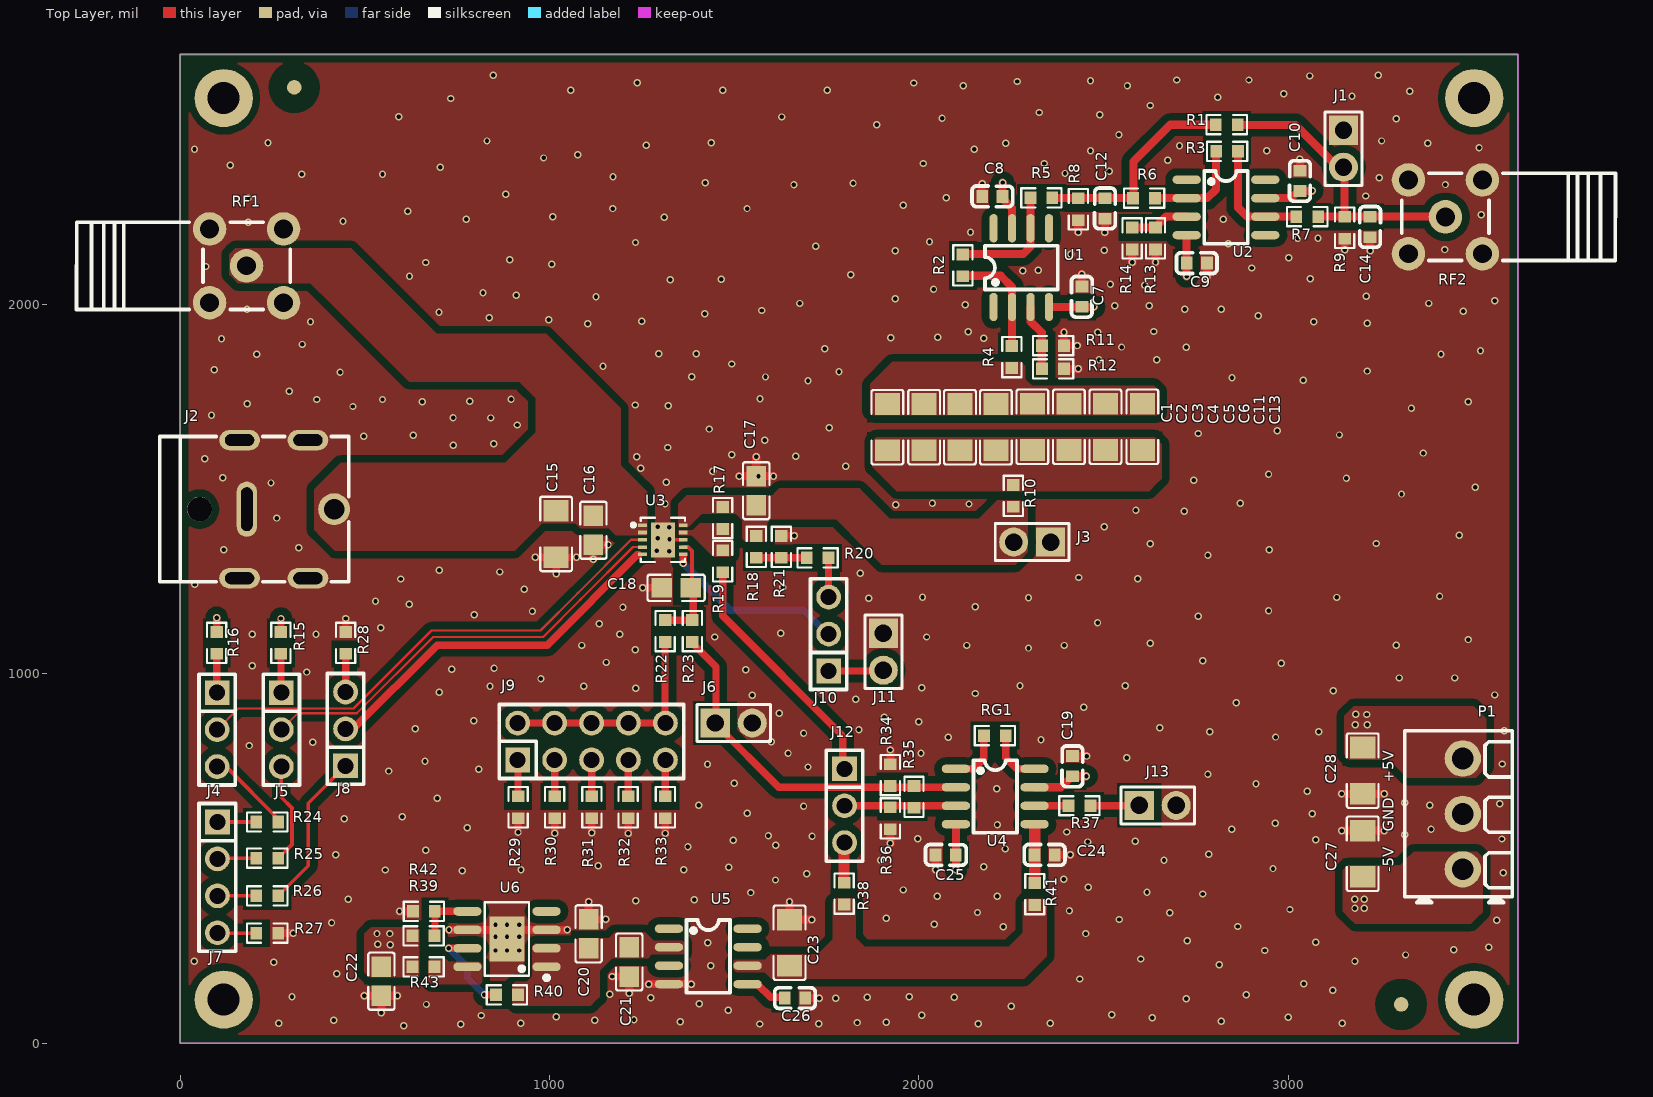
[diagram p0: Top Layer view]
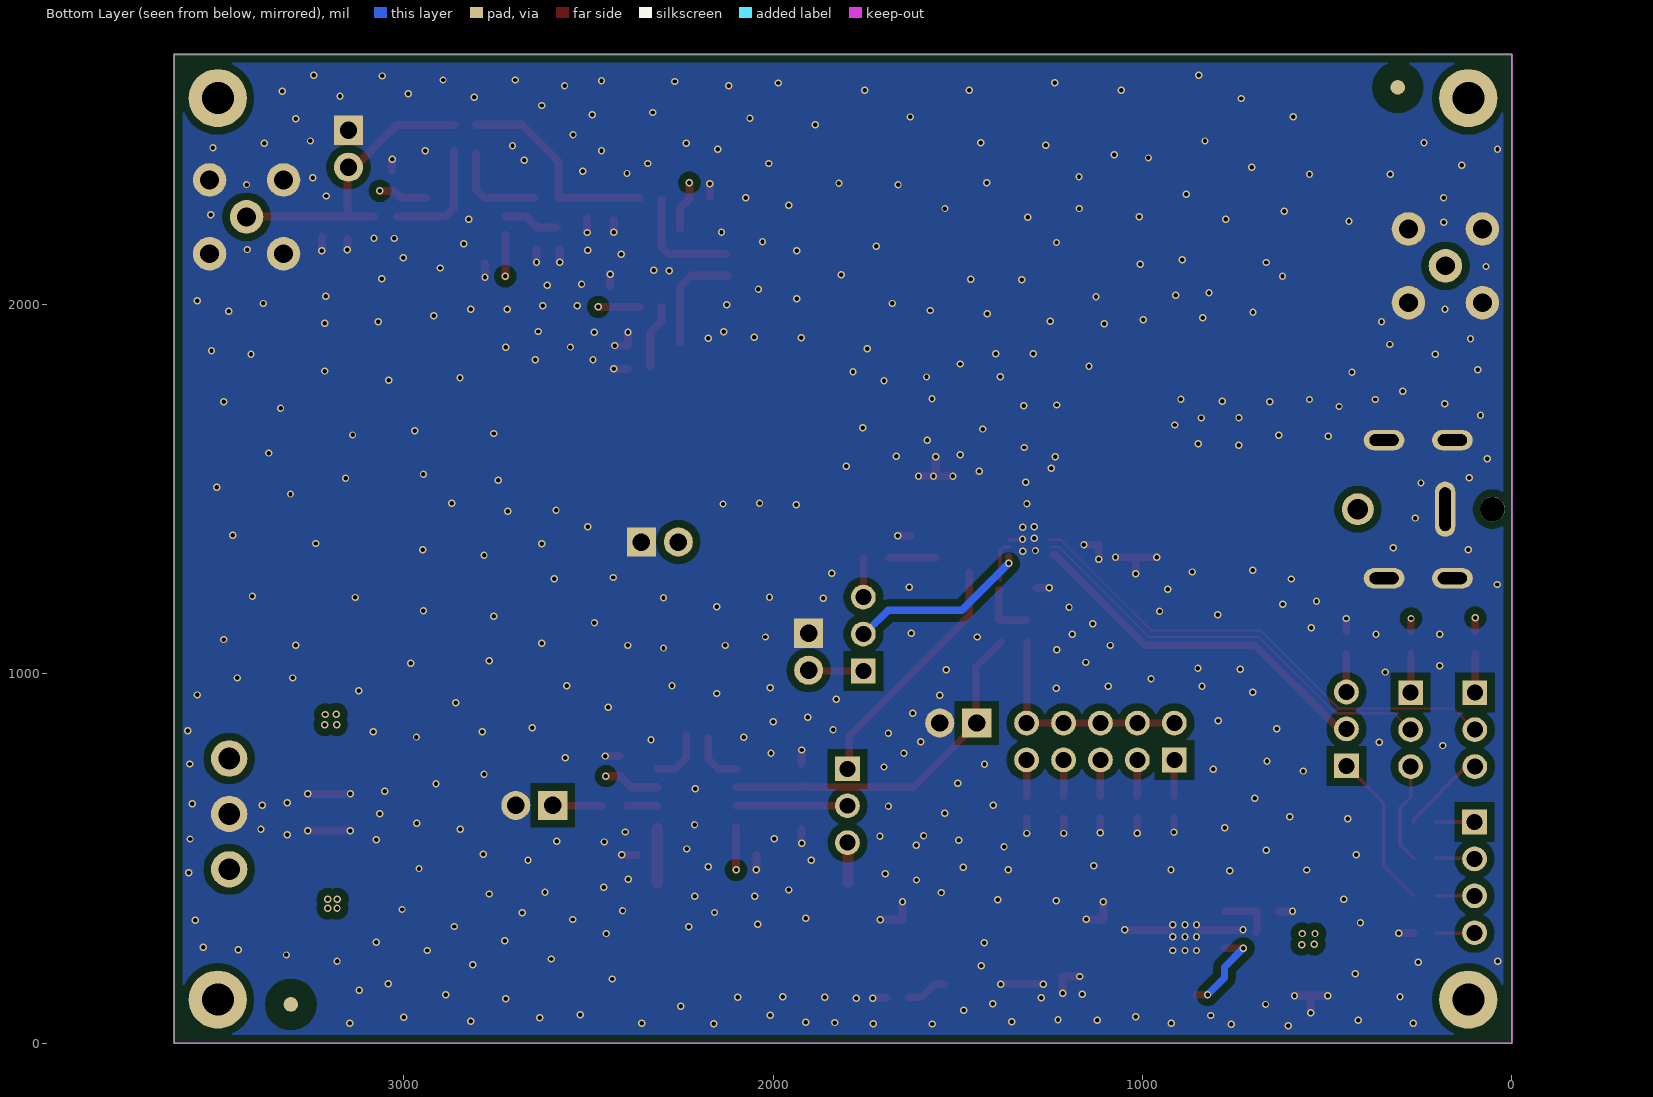
[diagram p1: Bottom Layer view, seen from below]
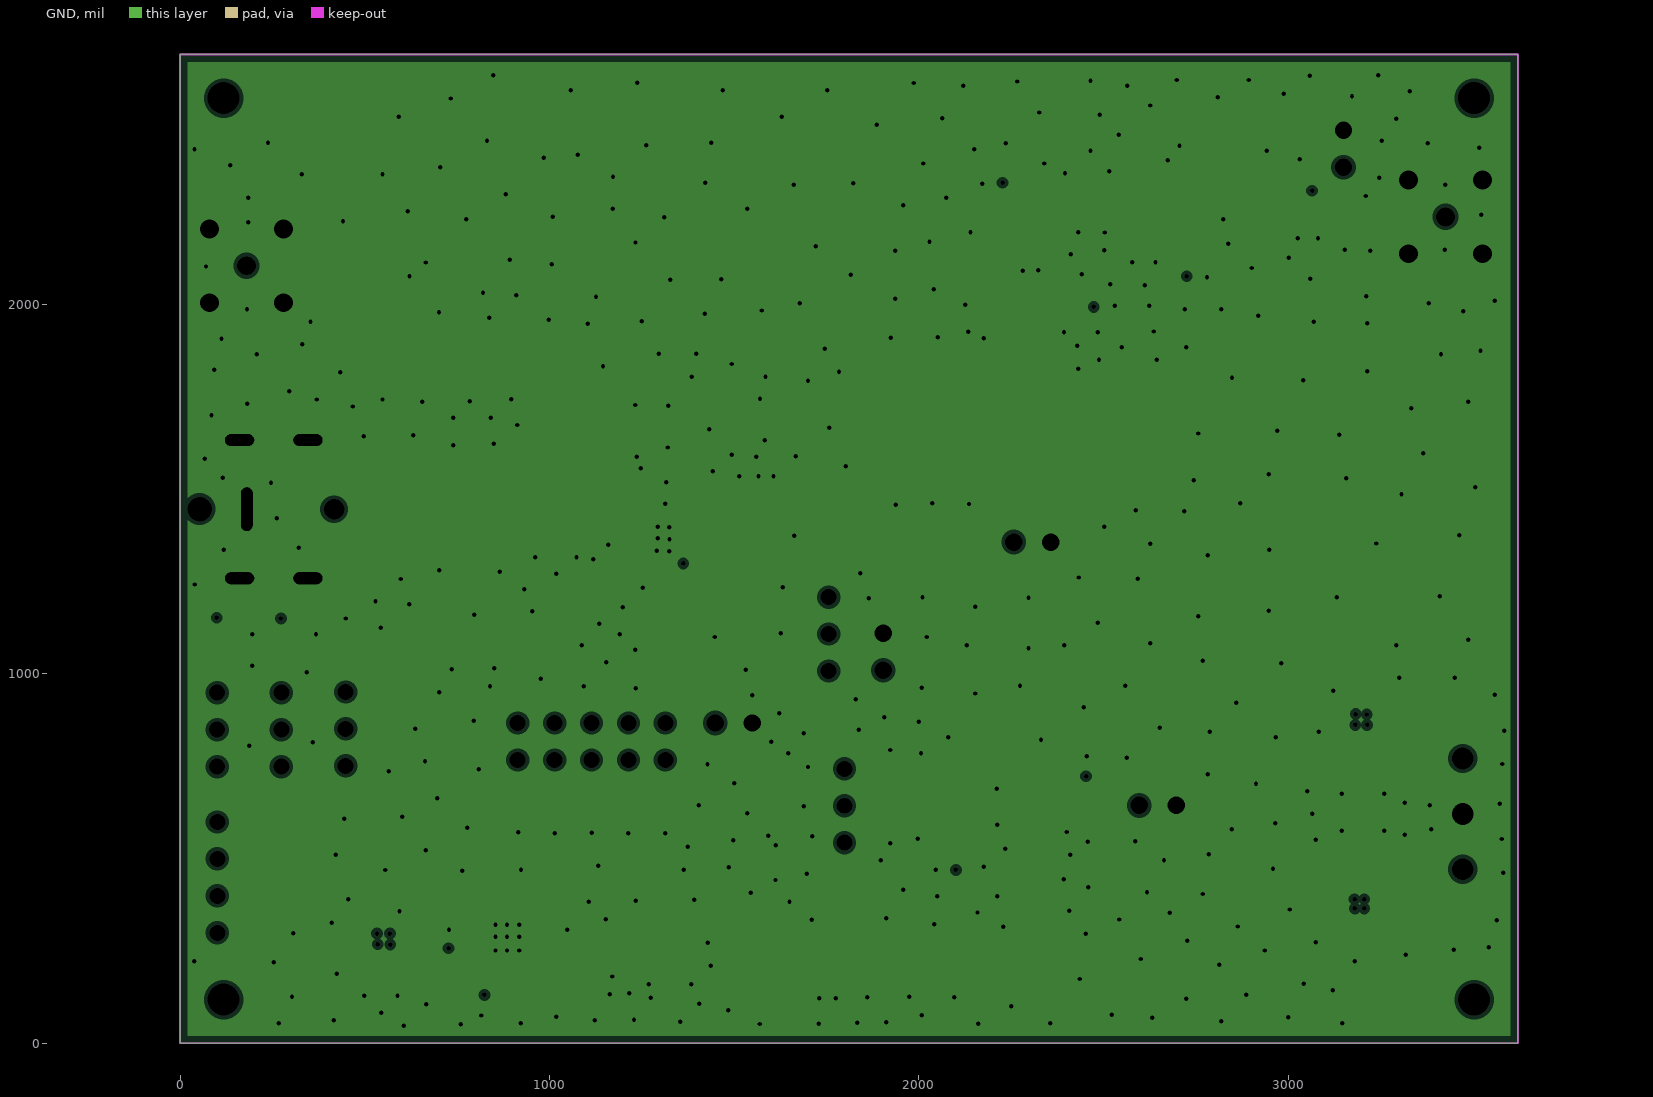
[diagram p2: GND, clearances drawn from the general rule]
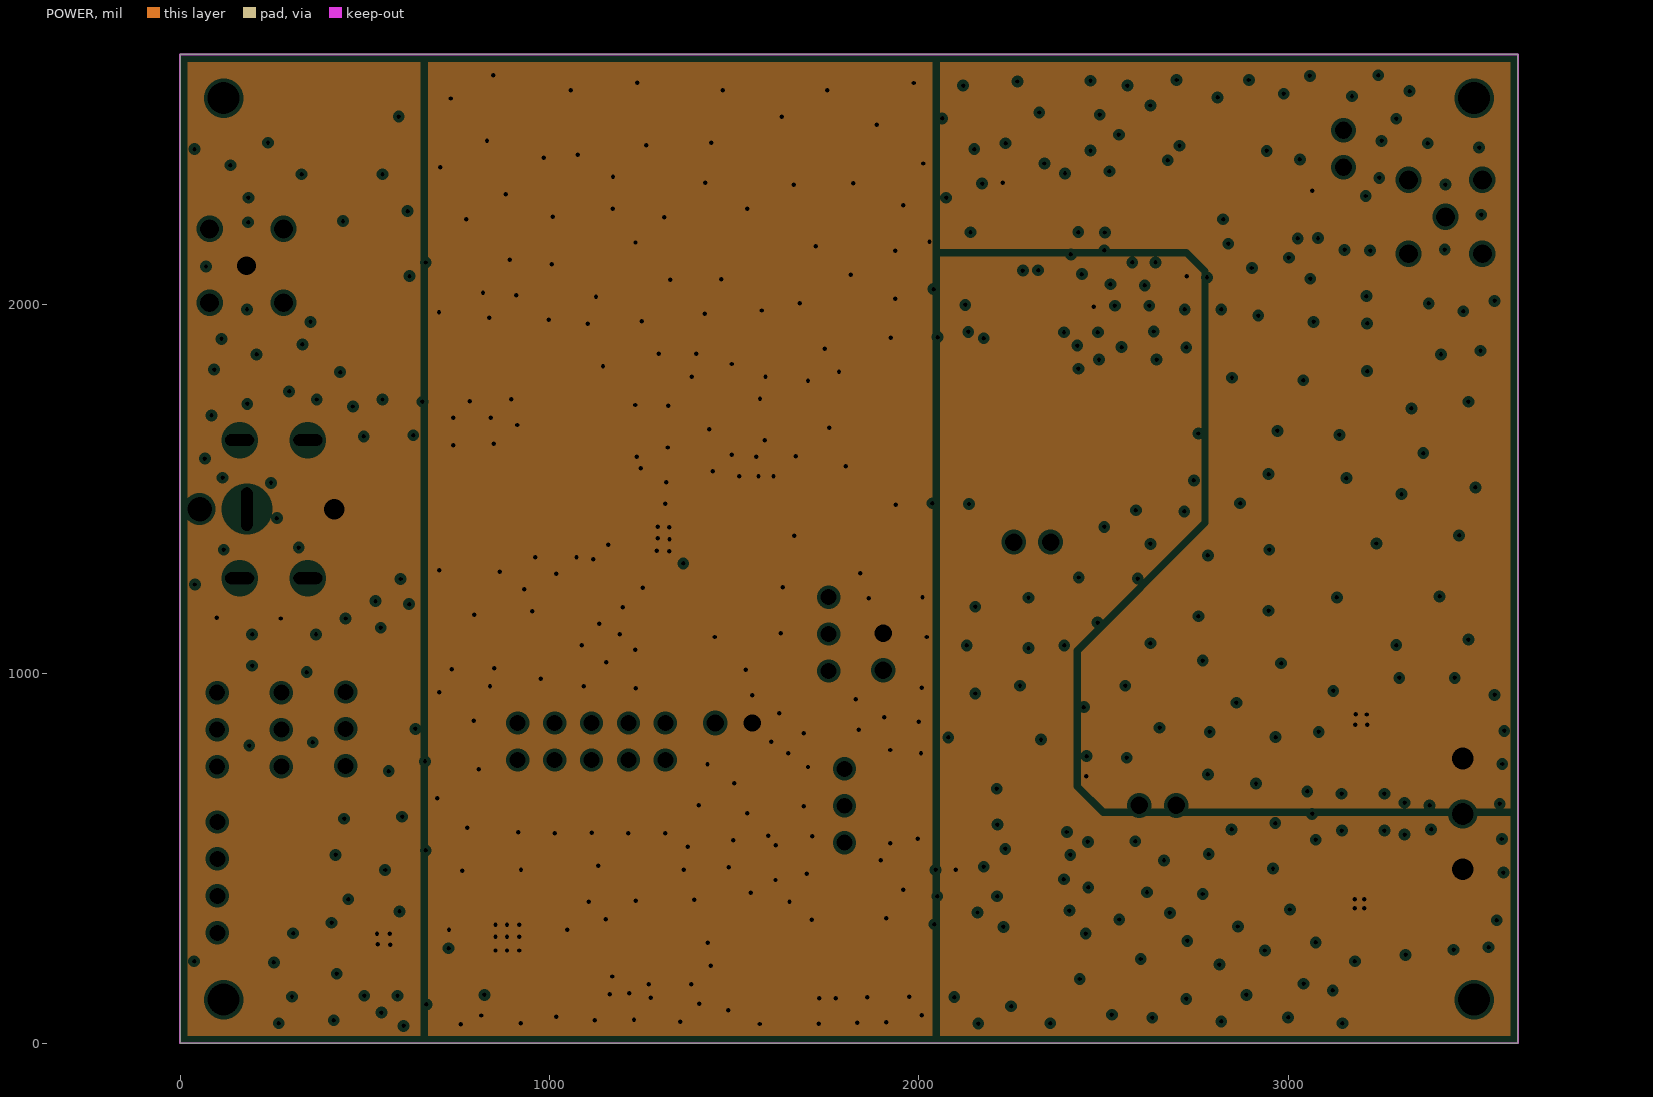
[diagram p3: POWER, clearances drawn from the general rule]
# Altium PCB MISC75514.PcbDoc
Units mil, origin at the board's own origin, x right, y up, seen from the top; angles counter-clockwise.
Board outline 3622.05 x 2677.17 mil, 4 copper layers (Top Layer, GND, POWER, Bottom Layer); 94 components, 55 nets, 263 pads, 522 vias.

## Layer stack, top to bottom (the 12.6 mil dielectric is the usual default, probably not edited)
Top Layer: signal copper 1.4
Dielectric: core 12.6, FR-4, Dk 4.8
GND: plane copper 1.4, net GND
Dielectric: prepreg 12.6, FR-4, Dk 4.8
POWER: plane copper 1.4
Dielectric: core 12.6, FR-4, Dk 4.8
Bottom Layer: signal copper 1.4

## Board outline
0,0 3622.05,0 3622.05,2677.17 0,2677.17

## Design rules (kind name [scope] priority, off if disabled: settings)
Clearance Clearance_3 [HASPAD('FREE-MARK')] p1: gap=50
Clearance Clearance_2 [INPOLYGON] p2: gap=6
Clearance [All] p3: gap=6
DiffPairsRouting [All] p1: maxlimit=6 minlimit=6 mostfreqgap=6 maxuncoupledlength=500
HoleSize [All] p1: absolutevalues=TRUE maxlimit=500 minlimit=1 maxpercent=80.000 minpercent=20.000
HoleToHoleClearance [All] p1: gap=0 allowstackedmicrovias=TRUE
MinimumSolderMaskSliver [All] p1: minsoldermaskwidth=0
PlaneClearance [All] p1: clearance=10
PlaneConnect [All] p1: planeconnectstyle=Direct reliefexpansion=20 reliefentries=4 reliefconductorwidth=10 reliefairgap=10
PolygonConnect [All] p1: connectstyle=Direct reliefconductorwidth=10 reliefentries=4 polygonreliefangle="90 Angle"
RoutingVias [All] p1: holewidth=12 width=20 viastyle="Through Hole" minholewidth=12 minwidth=20 maxholewidth=12 maxwidth=20
SilkToSilkClearance [All] p1: silktosilkclearance=0
SilkscreenOverComponentPads [All] p1: minsilkscreentomaskgap=0
SolderMaskExpansion [All] p1: expansion=4
Width [All] p1: maxlimit=40 minlimit=6 preferedwidth=6
20 further rules are at their usual default settings.

## Components (designator, comment, footprint, x,y, rotation, side; value= is the part's Value field where it differs from the comment)
C1 "GRM31CR60J227ME11L" C1206 1915,1668 r270 top
C2 "GRM31CR60J227ME11L" C1206 2014.55,1668.05 r270 top
C3 "GRM31CR60J227ME11L" C1206 2111.55,1668.05 r270 top
C4 "GRM31CR60J227ME11L" C1206 2209,1668 r270 top
C5 "22uF/35V" C1206 2307.55,1669.05 r270 top
C6 "22uF/35V" C1206 2406.55,1669.05 r270 top
C7 "100n/50V" C0603 2441.53,2021.35 r90 top
C8 "100n/50V" C0603 2199,2293 r180 top
C9 "100n/50V" C0603 2752.89,2112.05 r0 top
C10 "100n/50V" C0603 3032,2335 r90 top
C11 "22uF/35V" C1206 2505.55,1669.05 r270 top
C12 "100P/50V" C0603 2503.89,2260.05 r270 top
C13 "22uF/35V" C1206 2605.55,1669.05 r270 top
C14 "100P/50V" C0603 3221.89,2210.05 r270 top
C15 "22uF/35V" C1206 1018,1379 r90 top
C16 "4.7u/35V" C0805 1119,1389 r90 top
C17 "4.7u/35V" C0805 1560,1496 r270 top
C18 "4.7u/35V" C0805 1343,1233 r0 top
C19 "100n/50V" C0603 2416,750 r90 top
C20 "4.7u/35V" C0805 1106,296 r270 top
C21 "4.7u/35V" C0805 1216,220 r90 top
C22 "4.7u/35V" C0805 545,168 r90 top
C23 "22uF/35V" C1206 1650,272 r90 top
C24 "100n/50V" C0603 2341,510 r0 top
C25 "100n/50V" C0603 2073,510 r180 top
C26 "100n/50V" C0603 1665,122 r0 top
C27 "22uF/35V" C1206 3202,513 r270 top
C28 "22uF/35V" C1206 3202,738 r90 top
J1 "PZ254V-11-02P" HDR-TH_2P-P2.54-V-M 3150,2422 r270 top
J2 "HX DC007B-2.5" DC-IN-TH_HX-DC007B-2.5 289,1446 r0 top
J3 "PZ254V-11-02P" HDR-TH_2P-P2.54-V-M 2307,1357 r180 top
J4 "PZ254V-11-03P_C2937625" HDR-TH_3P-P2.54-V-M 100.21,849 r270 top
J5 "PZ254V-11-03P_C2937625" HDR-TH_3P-P2.54-V-M 274,849 r270 top
J6 "PZ254V-11-02P" HDR-TH_2P-P2.54-V-M 1499,867 r0 top
J7 "PZ254V-11-04P_C2691448" HDR-TH_4P-P2.54-V-M 101,449 r270 top
J8 "PZ254V-11-03P_C2937625" HDR-TH_3P-P2.54-V-M 448,851 r90 top
J9 "PZ254V-12-10P" HDR-TH_10P-P2.54-V-M-R2-C5-S2.54 1114,817 r0 top
J10 "PZ254V-11-03P_C2937625" HDR-TH_3P-P2.54-V-M 1756,1108 r90 top
J11 "PZ254V-11-02P" HDR-TH_2P-P2.54-V-M 1904,1060 r270 top
J12 "PZ254V-11-03P_C2937625" HDR-TH_3P-P2.54-V-M 1799,643 r270 top
J13 "PZ254V-11-02P" HDR-TH_2P-P2.54-V-M 2647,644 r0 top
P1 "DB125-3.81-3P-GN-S" CONN-TH_3P-P3.81_L7.4-W11.4 3473,621 r90 top
R1 "NC" R0603 2833.89,2487.05 r180 top
R2 "990R/1%" R0603 2119.55,2106.05 r270 top
R3 "990R/1%" R0603 2834.89,2415.05 r180 top
R4 "100R/1%" R0603 2252,1858 r90 top
R5 "0R/1%" R0603 2331.89,2289.05 r0 top
R6 "100R/1%" R0603 2609.89,2288.05 r0 top
R7 "0R/1%" R0603 3051.89,2238.05 r0 top
R8 "NC" R0603 2431.89,2258.05 r90 top
R9 "NC" R0603 3152.89,2208.05 r90 top
R10 "0R/1%" R0603 2256,1482 r270 top
R11 "100R/1%" R0603 2363.55,1889.05 r180 top
R12 "990R/1%" R0603 2363.55,1826.05 r180 top
R13 "100R/1%" R0603 2640.89,2179.05 r90 top
R14 "990R/1%" R0603 2577.89,2179.05 r90 top
R15 "200K/1%" R0603 273,1084 r90 top
R16 "1K/1%" R0603 99,1084 r90 top
R17 "0R/1%" R0603 1469,1422 r270 top
R18 "453K/1%" R0603 1560,1344 r270 top
R19 "0R/1%" R0603 1469,1305 r270 top
R20 "0R/1%" R0603 1726,1314 r180 top
R21 "49.9K/1%" R0603 1628,1344 r90 top
R22 "0R/1%" R0603 1313,1116 r270 top
R23 "0R/1%" R0603 1387,1116 r270 top
R24 "0R/1%" R0603 236,599 r180 top
R25 "0R/1%" R0603 236,501 r180 top
R26 "0R/1%" R0603 236,399 r180 top
R27 "0R/1%" R0603 236,298 r180 top
R28 "499R/1%" R0603 448,1084 r270 top
R29 "9K/1%" R0603 915,639 r90 top
R30 "18K/1%" R0603 1014,639 r90 top
R31 "25K/1%" R0603 1115,639 r90 top
R32 "30K/1%" R0603 1213,639 r90 top
R33 "50K/1%" R0603 1314,639 r90 top
R34 "NC" R0603 1923,726 r90 top
R35 "NC" R0603 1987,667 r270 top
R36 "NC" R0603 1923,609 r270 top
R37 "0R/1%" R0603 2435,643 r0 top
R38 "0R/1%" R0603 1798,405 r90 top
R39 "100K/1%" R0603 659,291 r180 top
R40 "100K/1%" R0603 885,131 r0 top
R41 "0R/1%" R0603 2314,404 r90 top
R42 "100K/1%" R0603 660,357 r0 top
R43 "0R/1%" R0603 659,207 r0 top
RF1 "KH-SMA-K513-G" ANT-TH_KH-SMA-K513-G 180,2105 r0 top
RF2 "KH-SMA-K513-G" ANT-TH_KH-SMA-K513-G 3425.89,2237.58 r180 top
RG1 "505R/1%" R0603 2206,833 r180 top
U1 "OPA211IDR" SOIC-8_L5.0-W4.0-P1.27-LS6.0-BL 2277.55,2100.05 r0 top
U2 "OPA211IDR" SOIC-8_L5.0-W4.0-P1.27-LS6.0-BL 2831.89,2263.05 r270 top
U3 "DU3042" WSON-10_L3.0-W3.0-P0.50-BL-EP 1307,1363 r270 top
U4 "INA828IDR" SOIC-8_L5.0-W4.0-P1.27-LS6.0-BL 2207,668 r270 top
U5 "REF5025AIDR" SOIC-8_L5.0-W4.0-P1.27-LS6.0-BL 1430,235 r270 top
U6 "ADP7104ARDZ-5.0-R7" SOIC-8_L4.9-W3.9-P1.27-LS6.0-BL-EP 885,282 r90 top

## Footprints (in the part's own frame and the unit in brackets; to place one, negate y for a bottom-side part, rotate by r counter-clockwise, add the part's x,y. Pads: shape width x height; smd on the part's side, far side on the other; paste and mask are expansions set on the pad)
ANT-TH_KH-SMA-K513-G [mm]
  round 2.3 hole 1.3 paste+0.051: 1(-2.54,-2.54) 2(-2.54,2.54) 3(2.54,2.54) 4(2.54,-2.54) 5(0,0)
  silkscreen extent -11.7,-3 3,3
C0603 [mm]
  rect 0.8x0.9 smd: 1(-0.7,0) 2(0.7,0)
  silkscreen extent -1.41,-0.71 1.39,0.72
C0805 [mm]
  rect 1.41x1.35 smd paste-100 mask+0.051: 1(-1,0) 2(1,0)
  silkscreen extent -1.96,-0.9 1.96,0.9
C1206 [mm]
  rect 1.485x1.728 smd paste-100 mask+0.051: 1(-1.593,0) 2(1.593,0)
  silkscreen extent -2.56,-1.09 2.56,1.09
CONN-TH_3P-P3.81_L7.4-W11.4 [mm]
  round 2.5 hole 1.5 paste+0.051: 1(-3.81,0) 2(0,0) 3(3.81,0)
  silkscreen extent -6.1,-3.4 5.71,4
DC-IN-TH_HX-DC007B-2.5 [mm]
  round 1.7 hole 1.7 unplated: 0(-6,0)
  round 2.2 hole 1.4: 1(3.25,0)
  oval 1.4x3.8 hole 0.8 slot 3 at 90 deg: 2(-2.75,0)
  oval 2.8x1.4 hole 0.8 slot 2 at 0 deg: 3(-3.25,-4.75) 3(-3.25,4.75) 3(1.45,-4.75) 3(1.45,4.75)
  silkscreen extent -8.75,-5 4.25,5
HDR-TH_2P-P2.54-V-M [mm]
  rect 2x2 hole 1.2 paste+0.051: 1(-1.27,0)
  round 2 hole 1.2 paste+0.051: 2(1.27,0)
  silkscreen extent -2.54,-1.27 2.54,1.27
HDR-TH_3P-P2.54-V-M [mm]
  rect 1.7x1.7 hole 1.1 paste+0.051: 1(-2.54,0)
  round 1.7 hole 1.1 paste+0.051: 2(0,0) 3(2.54,0)
  silkscreen extent -3.81,-1.25 3.81,1.25
HDR-TH_4P-P2.54-V-M [mm]
  rect 1.7x1.7 hole 1.1 paste+0.051: 1(-3.81,0)
  round 1.7 hole 1.1 paste+0.051: 2(-1.27,0) 3(1.27,0) 4(3.81,0)
  silkscreen extent -5.08,-1.27 5.08,1.27
HDR-TH_10P-P2.54-V-M-R2-C5-S2.54 [mm]
  rect 1.7x1.7 hole 1.1 paste+0.051: 1(-5.08,-1.27)
  round 1.7 hole 1.1 paste+0.051: 2(-5.08,1.27) 3(-2.54,-1.27) 4(-2.54,1.27) 5(0,-1.27) 6(0,1.27) 7(2.54,-1.27) 8(2.54,1.27) 9(5.08,-1.27) 10(5.08,1.27)
  silkscreen extent -6.35,-2.54 6.35,2.54
R0603 [mil]
  rect 31.75x34.02 smd paste-3937.01 mask+2: 1(-29.66,0) 2(29.66,0)
  silkscreen extent -55,-26 55,26
SOIC-8_L4.9-W3.9-P1.27-LS6.0-BL-EP [mm]
  oval 0.602x1.941 smd paste+0.051: 1(-1.905,-2.721) 2(-0.635,-2.721) 3(0.635,-2.721) 4(1.905,-2.721) 5(1.905,2.721) 6(0.635,2.721) 7(-0.635,2.721) 8(-1.905,2.721)
  rect 3.098x2.41 smd paste+0.051: 9(0,0)
  silkscreen extent -2.81,-2.87 2.53,1.52
SOIC-8_L5.0-W4.0-P1.27-LS6.0-BL [mil]
  oval 22.38x76.78 smd paste+2: 1(-75,-106.5) 2(-25,-106.5) 3(25,-106.5) 4(75,-106.5) 5(75,106.5) 6(25,106.5) 7(-25,106.5) 8(-75,106.5)
  silkscreen extent -98,-59 98,59
WSON-10_L3.0-W3.0-P0.50-BL-EP [mm]
  rect 0.25x0.6 smd paste+0.051: 1(-1.001,-1.4) 2(-0.5,-1.4) 3(0,-1.4) 4(0.5,-1.4) 5(1.001,-1.4) 6(1.001,1.4) 7(0.5,1.4) 8(0,1.4) 9(-0.5,1.4) 10(-1.001,1.4)
  rect 2.4x1.65 smd paste+0.051: 11(0,0)
  silkscreen extent -1.52,-2.14 1.52,1.52

## Part data
C1 C2 C3 C4 C5 C6 C11 C13 C15 C16 C17 C18 C20 C21 C22 C23 C27 C28: library part C, "SMD capacitor"
C7 C8 C9 C10 C12 C14 C19 C24 C25 C26: library part 1uF
P1: library part WJ124-3.81-3P
R1 R2 R3 R4 R5 R6 R7 R8 R9 R10 R11 R12 R13 R14 R15 R16 R17 R18 R19 R20 R21 R22 R23 R24 R25 R26 R27 R28 R29 R30 R31 R32 R33 R34 R35 R36 R37 R38 R39 R40 R41 R42 R43 RG1: library part R, "SMD resistor"
U1 U2: library part INA828IDR
U3: library part DAC53202RTER, "No Description Available"

## Free pads (board coordinates)
  round 157.48 hole 86.61: 3(118.11,2559.06) 4(118.11,118.11) 5(3503.94,118.11) 6(3503.94,2559.06)
  round 39.37 smd mask+39.37: MARK(309,2588) MARK(3306,105)
  round 39.37 smd far side mask+39.37: MARK(309,2588) MARK(3306,105)

## Via types
v1: diameter 20, hole 12, Top Layer to Bottom Layer, 522 vias

## Nets (pads, with @x,y where several pads share a name; then routed paths per layer and width w, separated by ;. In a path a pad name is that pad's centre, name@x,y a point inside that pad or via, vN(x,y) a via of type N, cw(c..) or ccw(c..) an arc to the next point about the centre after c; other vN are vias at no path point)
+5V: C8.1 C10.1 C19.1 C28.2 P1.3 U1.7 U2.7 U4.7 | length 420.8
  Top Layer w22: v1(2227,2330) 2227,2287 2252.55,2261.45 U1.7 ; U4.7 2385,693 2415,723 v1(2453,723) ; U2.7 3008.05,2288.05 3028,2308 v1(3065,2308)
  other v1: 3182,862 3214,862 3213,890 3183,891
-5V: C7.1 C9.1 C25.1 C27.2 P1.1 U1.4 U2.4 U4.4 | length 338.6
  Top Layer w22: v1(2100.56,469.44) C25.1 U4.4@2100.56,583.56 ; U1.4@2360.79,1993.79 C7.1 v1(2473.79,1993.79) ; v1(2725.39,2076.61) U2.4
  other v1: 3181,365 3206,365 3180,390 3206,390
GND: C7.2 C8.2 C9.2 C10.2 C12.2 C14.2 C15.1 C16.1 C17.1 C18.1 C19.2 C20.1 C21.1 C22.1 C23.2 C24.2 C25.2 C26.2 C27.1 C28.1 J1.1 J2.2 J2.3 J3.1 J6.2 J11.1 J13.2 P1.2 R8.1 R9.1 R11.1 R12.1 R13.1 R14.1 R21.2 R27.1 R28.1 R29.1 R30.1 R31.1 R32.1 R33.1 R34.2 R36.2 R42.1 RF1.1 RF1.2 RF1.3 RF1.4 RF2.1 RF2.2 RF2.3 RF2.4 U3.8 U3.11 U5.4 U6.3 U6.6 U6.9 | length 2488
  Top Layer w10: U3.11@1338,1363 U3.8
  Top Layer w20: R28.1 v1(448,1150) ; v1(915,571) R29.1 ; v1(961.7,1316.3) C15.1 ; v1(1014,569) R30.1 ; v1(1018,1271) C15.1 ; v1(1073.3,1316.3) C15.1 ; v1(1115,570) R31.1 ; v1(1119,1310) C16.1 v1(1158.63,1349.63) ; v1(1213,568) R32.1 ; v1(1253,1233) C18.1@1288,1233 ; v1(1314,568) R33.1 ; R21.2 v1(1662.34,1373.66)
  Top Layer w22: R27.1 v1(306,298) ; v1(498.37,128.63) C22.1 ; v1(545,83) C22.1 ; v1(588.63,128.63) C22.1 ; v1(594,357) R42.1 ; v1(728,307) U6.6 U6.9@841,307 ; U6.9@928,307 U6.3 v1(1048,307) ; v1(1106,383) C20.1 v1(1152.37,335.37) ; v1(1169.63,180.63) C21.1 v1(1216,135) ; v1(1269,160) U5.4 v1(1384,160) ; v1(1513.37,1535.37) C17.1 ; v1(1560,1588) C17.1 ; v1(1606.63,1535.37) C17.1 ; v1(1650,383) C23.2 v1(1710.3,334.7) ; C26.2 v1(1730,122) ; v1(1923,541) R36.2 ; R34.2 v1(1923,794) ; v1(2045.44,469.44) C25.2 ; C8.2 v1(2171.44,2327.44) ; C24.2 v1(2410,510) ; R12.1 v1(2432.05,1826.05) ; v1(2393.21,1925.21) R11.1 v1(2428.95,1889.05) ; C19.2 v1(2454.44,777.56) ; v1(2431.89,2196.11) R8.1 ; C7.2 v1(2441.53,2082.53) ; v1(2503.89,2195.11) C12.2 ; v1(2577.89,2114.11) R14.1 ; v1(2640.89,2114.11) R13.1 ; v1(2780.45,2073.45) C9.2 ; C10.2 v1(3032,2393) ; v1(3144.7,675.3) C28.1 v1(3260.7,675.3) ; v1(3145.7,575.7) C27.1 v1(3260.7,575.7) ; v1(3152.89,2148.11) R9.1 ; v1(3221.89,2146.11) C14.2
  other v1: 605,47 760,51 1569,52 1729,53 2161,53 267,54 922,54 2356,54 3147,54 1833,56 1912,57 1354,58 2819,59 416,62 1123,62 1229,64 2632,69 3000,70 1018,72 815,75 2008,76 2523,77 1484,89 2250,100 667,105 1406,107 2724,120 1775,122 1274,123 1860,124 2096,125 303,126 1974,126 2887,131 1163,133 3121,143 3042,161 2436,174 424,188 1437,210 2814,213 254,219 38,222 3181,222 2601,228 3318,239 854,251 885,251 918,251 2937,251 3448,253 3543,260 1429,272 3075,273 2727,277 854,288 885,288 918,288 2452,297 2229,315 2864,316 854,321 885,321 918,321 2042,322 410,326 3565,333 2543,335 1912,338 2680,353 2159,354 2408,359 3005,362 1234,386 1392,388 455,390 2050,398 2212,398 2769,404 1545,408 2618,409 1958,415 2459,422 1612,442 2393,444 1697,459 3583,462 764,467 555,469 923,470 1364,470 2959,473 1485,476 2176,478 1132,481 1897,495 2664,495 421,510 2785,512 665,522 2234,526 1375,532 1613,536 2458,545 2586,547 1498,550 3075,551 3579,553 1997,554 1711,560 1593,562 3315.52,565 2401,572 2847,579 3387,579 777,583 2213,592 2965,596 444,608 601,613 3065,621 1536,623 1688,642 1404,644 3383,644 3573,648 3315.52,651 696,663 3052,682 2211,689 2913,703 1500,704 2783,728 565,737 809,742 1700,748 1428,755 3580,756 663,763 2563,773 1646,785 2006,785 187,806 359,815 1601,816 2331,822 2080,828 2966,829 1688,839 2788,843 3083,843 3585,845.81 1838,849 637,851 2652,854 2000,870 795,873 1906,883 1622,893 2447,910 2860,922 1829,931 1549,942 3559,943 2153,947 702,950 3122,954 1234,961 2008,962 839,967 1093,967 2274,968 2559,968 977,987 3301,989 3451,989 343,1005 1531,1011 735,1013 850,1015 195,1022 2981,1029 1154,1031 2769,1036 1232,1065 2297,1070 1087,1077 2130,1077 2394,1077 3293,1078 2627,1083 3488,1093 1448,1100 2021,1100 195,1107 368,1107 1190,1107 1626,1110 543,1125 1135,1136 2484,1139 2757,1156 796,1160 954,1170 2947,1171 1199,1180 2153,1182 620,1189 529,1197 1865,1205 2297,1206 3132,1207 2010,1208 3410,1210 932,1229 1632,1235 40,1242 597,1257 2593,1258 2433,1261 1842,1272 865,1276 702,1281 2783,1321 1324,1332 1290,1334 118,1336 2949,1336 321,1342 2627,1352 3239,1353 1325,1365 1293,1367 3463,1375 1324,1397 1293,1398 2502,1398 262,1422 2719,1440 2588,1443 1938,1458 2136,1460 1313,1461 2037,1462 2870,1462 3307,1487 3507,1505 246,1517 1316,1519 2745,1524 3158,1530 115,1531 1566,1535 2947,1541 1442,1549 1247,1557 1802,1562 67,1583 1236,1588 1667,1589 1494,1593 3366,1598 1320,1613 740,1619 849,1623 1583,1633 497,1643 631,1646 3139,1647 2757,1651 2971,1658 1433.18,1663 1758,1667 913,1674 841,1693 739,1694 85,1700 3334,1719 468,1724 1322,1726 1232,1728 182,1731 656,1737 3488,1737 784,1738 370,1743 548,1743 896,1744 1570,1745 295,1765 1700,1794 3041,1795 2848,1802 1585,1804 1385,1805 433,1817 1784,1818 3214,1820 92,1824 1145,1833 1494,1839 2488,1851 2644,1851 207,1865 3414,1865 1296,1867 1398,1867 3521,1875 1745,1880 2724,1884 2549,1885 331,1892 112,1907 2176,1909 1924,1910 2051,1912 2485,1925 2134,1926 2636,1927 1104,1948 3214,1949 353,1953 3069,1953 1250,1955 998,1959 837,1964 2919,1970 1421,1975 701,1979 3474,1982 1575,1984 181,1986.89 2720,1987 2819,1987 2531,1997 2624,1997 2126,1999 1678,2003 3381,2003 3559,2010 1936,2016 1126,2021 3212,2023 910,2025 820,2032 2040,2042 2612,2052 2519,2055 1327,2067 1465,2068.18 3060,2070 621,2077 1816,2081 2282,2092 2323,2093 2902,2099 70,2103 1006,2109 665,2114 893,2121 3002,2127 2412,2136 1936,2146 2502,2147 3424,2149 1721,2158 2838,2164.62 1233,2168 2029,2170 3026,2179 3081,2180 2140,2196 184,2223.11 441,2226 775,2231 2824,2231 1311,2236 1009,2238 3523,2243 616,2253 1171,2260 1535,2260 1958,2269 185,2289 2074,2289 3210,2294 882,2299 1662,2324 3426,2325 1822,2328 1422,2330 3247,2343 1172,2346 329,2353 548,2353 2396,2355 2516,2361 704,2372 136,2377 2012,2382 2340,2382 2674,2391 984,2397 1077,2406 2942,2416 2465,2417 39,2421 2150,2421 3517,2425 2706,2430 1262,2431 2235,2437 3378,2437 238,2438 1438,2438 831,2443 3253,2443 2542,2460 1886,2487 3293,2503 2063,2504 1629,2508 592,2509 2490,2514 2326,2520 2627,2539 733,2558 2809,2561 3173,2564 2988,2571 3329,2578 1058,2580 1469,2580 1752,2580 2120,2593 2565,2593 1986,2600 1238,2601 2267,2604 2465,2606 2698,2608 2894,2608 3059,2619 848,2621 3244,2621
NetC1_1: C1.1 C2.1 C3.1 C4.1 C5.1 C6.1 C11.1 C13.1 R4.1
NetC1_2: C1.2 C2.2 C3.2 C4.2 C5.2 C6.2 C11.2 C13.2 R10.1
NetC12_1: C12.1 R1.2 R5.2 R6.1 R8.2 | length 589.3
  Top Layer w22: R5.2 R6.1@2580.95,2289.05 ; R6.1@2582,2288 R6.1@2581,2289 ; R1.2 2681.05,2487.05 2581,2387 R6.1@2581,2294 ; R6.1@2580.95,2289.05 R6.1@2581,2289 ; R6.1@2580.95,2289.05 2580,2290 2580,2293 R6.1@2581,2294 ; R6.1@2581,2289 R6.1@2581,2294
NetC14_1: C14.1 J1.2 R1.1 R7.2 R9.2 RF2.5 | length 789.6
  Top Layer w22: R1.1 R1.1@2867,2487.05 ; R1.1@2867,2486 3020,2486 J1.2@3135,2371 ; R7.2 R9.2@3152.89,2238.05 ; J1.2@3136,2372 J1.2@3143,2365 ; R9.2 R9.2@3152.89,2238.05 ; J1.2@3160,2371 3152.89,2363.89 R9.2@3152.89,2238.05 ; RF2.5@3405.95,2238.05 R9.2@3152.89,2238.05
NetC17_2: C17.2 J3.2 R10.2 R17.1 R18.1 U3.10
NetC18_2: C18.2 R22.1 R23.1 U3.7 | length 261
  Top Layer w11: U3.7 1375.7,1343.3 1386,1333 C18.2@1386,1256
  Top Layer w20: R22.1 1384,1145.66 R23.1@1386.34,1145.66 ; C18.2@1386,1228 C18.2@1386.34,1227.66 ; R23.1@1389,1146 1389,1194 C18.2@1389,1228
NetC24_1: C24.1 R41.2 U4.5 | length 147.3
  Top Layer w30: R41.2 2314,581
NetC26_1: C26.1 U5.5 | length 110.4
  Top Layer w20: U5.5 1563,160 1599,124 C26.1@1632,124
NetJ4_1: J4.1 R16.1 | length 104.1
  Top Layer w20: J4.1@99,950.21 R16.1
NetJ4_2: J4.2 U3.3 | length 1368.2
  Top Layer w6: J4.2 157.75,906.54 469.54,906.54 680.5,1117.5 975.5,1117.5 1078,1220 ; 1075.5,1217.5 1078,1220 ; U3.3 U3.3 1221,1363 1078,1220
NetJ4_3: J4.3 R24.1 | length 232.5
  Top Layer w10: J4.3 124,749 265.66,607.34 R24.1
NetJ5_1: J5.1 R15.1 | length 104.3
  Top Layer w20: J5.1@273,950 R15.1
NetJ5_2: J5.2 U3.4 | length 1185.5
  Top Layer w6: J5.2 318.46,893.46 478.46,893.46 685,1100 983,1100 1085,1202 ; 1083,1200 1085,1202 ; U3.4 1226.31,1343.31 1085,1202
NetJ5_3: J5.3 R25.1 | length 275.5
  Top Layer w10: R25.1 303,538.34 303,637 274,666 J5.3
NetJ6_1: J6.1 R23.2 R34.1 R35.1 U4.2 | length 965.4
  Top Layer w20: R23.2@1384,1086.34 1451,1019.34 1451,863 1621,693 1911,693 1914.34,696.34 R34.1 ; R34.1@1930,693 U4.2
NetJ7_1: J7.1 R24.2 | length 105.3
  Top Layer w10: J7.1 R24.2
NetJ7_2: J7.2 R25.2 | length 103.3
  Top Layer w10: J7.2@103,501 R25.2
NetJ7_3: J7.3 R26.2 | length 105.3
  Top Layer w10: J7.3 R26.2
NetJ7_4: J7.4 R27.2 | length 104.3
  Top Layer w10: J7.4@102,298 R27.2
NetJ8_1: J8.1 R26.1 | length 427.5
  Top Layer w10: R26.1 347,480.34 347,650 J8.1
NetJ8_2: J8.2 U3.5 | length 999.1
  Top Layer w6: U3.5@1242.14,1323.63 U3.5
  Top Layer w20: J8.2 469,851 696,1078 994,1078 1238.14,1322.14 U3.5@1242.14,1322.14
NetJ8_3: J8.3 R28.2 | length 103.3
  Top Layer w20: J8.3 R28.2
NetJ9_1: J9.1 R29.2 | length 76.3
  Top Layer w20: R29.2 J9.1@915,745
NetJ9_2: J9.2 J9.4 J9.6 J9.8 J9.10 R22.2 | length 600.3
  Top Layer w20: J9.2 J9.4 J9.6 J9.8 J9.10@1304,867 ; J9.10@1313,876 R22.2
NetJ9_3: J9.3 R30.2 | length 77.3
  Top Layer w20: R30.2 J9.3@1014,746
NetJ9_5: J9.5 R31.2 | length 84.3
  Top Layer w20: R31.2 1115,722 J9.5@1115,753
NetJ9_7: J9.7 R32.2 | length 81.3
  Top Layer w20: R32.2 J9.7@1213,750
NetJ9_9: J9.9 R33.2 | length 82.3
  Top Layer w20: R33.2 J9.9@1314,751
NetJ10_1: J10.1 J11.2 | length 144
  Top Layer w20: J10.1 J11.2@1900,1008
NetJ10_2: J10.2 U3.6 | length 479
  Top Layer w20: v1(1362.11,1299.11) 1362.11,1318
  Bottom Layer w20: v1(1362.11,1299.11) 1489.23,1172 1689,1172 J10.2@1746,1115
NetJ10_3: J10.3 R20.1 | length 84.3
  Top Layer w20: J10.3@1755.66,1229.66 R20.1
NetJ12_1: J12.1 R19.2 | length 651
  Top Layer w20: R19.2 1469,1157 1794,832 J12.1@1794,759
NetJ12_2: J12.2 R35.2 R36.1 U4.3 | length 292.2
  Top Layer w20: J12.2@1810,639 1814,643 U4.3
NetJ12_3: J12.3 R38.2 | length 107.3
  Top Layer w30: R38.2 J12.3@1798,542
NetJ13_1: J13.1 R37.2 | length 109.3
  Top Layer w20: R37.2 J13.1@2574,643
NetR2_1: R2.1 R5.1 U1.6 | length 310.6
  Top Layer w22: R2.1@2128,2137 2283,2137 2302.55,2156.55 U1.6 R5.1@2302.55,2284.55
NetR2_2: R2.2 R4.2 U1.2 | length 292.1
  Top Layer w22: R2.2@2122,2078 2222,2078 2252.55,2047.45 U1.2 R4.2@2252.55,1898.55
NetR3_1: R3.1 R7.1 U2.6 | length 325.6
  Top Layer w22: R3.1 2864.55,2262.45 2871,2256 ; 2865,2262 2871,2256 ; R7.1@3018.95,2238.05 U2.6 2888.95,2238.05 2871,2256
NetR3_2: R3.2 R6.2 U2.2 | length 266
  Top Layer w22: R6.2@2645.95,2288.05 U2.2 2781.05,2288.05 2805,2312 R3.2@2805,2409
NetR11_2: R11.2 R12.2 U1.3 | length 174.2
  Top Layer w22: U1.3 2302.55,1954.45 2333,1924 R12.2@2333,1832
NetR13_2: R13.2 R14.2 U2.3 | length 151.4
  Top Layer w22: R14.2@2586,2209 2640,2209 2669.05,2238.05 U2.3
NetR17_2: R17.2 R19.1 U3.9
NetR18_2: R18.2 R20.2 R21.1 | length 127.7
  Top Layer w20: R18.2 R21.1 R20.2@1687.66,1314.34
NetR37_1: R37.1 U4.6 | length 82.5
  Top Layer w20: U4.6 R37.1@2396,643
NetR39_1: R39.1 R42.2 U6.5 | length 145.5
  Top Layer w20: R39.1@694,301 690,305 690,357 U6.5
NetR40_1: R40.1 U6.7 | length 248.4
  Top Layer w20: v1(727,257) U6.7 ; v1(824,131) R40.1
  Bottom Layer w20: v1(727,257) 778,206 778,177 v1(824,131)
NetR43_2: R43.2 U6.8
NetRG1_1: RG1.1 U4.8 | length 150.7
  Top Layer w20: RG1.1 2235.66,772.34 2265,743 U4.8
NetRG1_2: RG1.2 U4.1 | length 143.7
  Top Layer w20: U4.1 2149,743 2176,770 RG1.2@2176,827
REF_2.5V: C23.1 R38.1 R41.1 U5.6
REF_5V: C20.2 C21.2 R40.2 U5.2 U6.1 U6.2
VIN: C15.2 C16.2 C22.2 J2.1 R15.2 R16.2 R39.2 R43.1 RF1.5 U3.1 U3.2 | length 74.7
  Top Layer w20: R16.2 v1(99,1152) ; R15.2 v1(273,1150)
  other v1: 569,267 535,268 533,297 568,297
pads on no net: J2.0 U1.1 U1.5 U1.8 U2.1 U2.5 U2.8 U5.1 U5.3 U5.7 U5.8 U6.4

## Polygon pours and split planes (outlines as drawn)
VIN on Top Layer "Bottom Layer-No Net" (solid, remove dead copper): 363,1472 363,1390 384,1369 419,1334 784,1334 906,1334 956,1384 980,1408 1024,1408 1070,1408 1078,1400 1083,1395 1123,1395 1161,1395 1168,1388 1180,1376 1248,1376 1262,1376 1264,1378 1265,1379 1265,1383 1265,1493 1232,1526 1193,1565 1193,1628 1193,1719 1037,1875 991,1921 826,1921 695,1921 601,2015 464,2152 220,2152 149,2152 144,2147 133,2136 133,2113 133,2081 142,2072 156,2058 200,2058 353,2058 410,2001 620,1791 900,1791 918,1791 933,1776 963,1746 963,1719 963,1654 940,1631 881,1572 712,1572 435,1572 378,1515 363,1500 363,1472
REF_5V on Top Layer "Bottom Layer-No Net" (solid, remove dead copper): 899,143 899,120 899,111 905,105 908,102 1098,102 1112,102 1123,113 1136,126 1136,152 1136,196 1157,217 1170,230 1212,230 1267,230 1276,239 1278,241 1321,241 1361,241 1363,243 1365,245 1365,250 1365,272 1361,276 1359,278 1347,278 1282,278 1266,294 1260,300 1227,300 1177,300 1165,288 1161,284 1124,284 1078,284 1067,273 1065,271 1021,271 962,271 957,266 954,263 954,257 954,182 947,175 938,166 927,166 908,166 904,162 899,157 899,143
NetC1_1 on Top Layer "Bottom Layer-No Net" (solid, remove dead copper): 1868,1785 1868,1710 1873,1705 1878,1700 1891,1700 2645,1700 2649,1704 2651,1706 2651,1714 2651,1766 2645,1772 2637,1780 2575,1780 2307,1780 2293,1794 2288,1799 2288,1816 2288,1834 2282,1840 2277,1845 2265,1845 1928,1845 1868,1785
NetC1_2 on Top Layer "Bottom Layer-No Net" (solid, remove dead copper): 1874,1602 1874,1561 1884,1551 1940,1495 2246,1495 2624,1495 2645,1516 2658,1529 2658,1554 2658,1622 2646,1634 2639,1641 2627,1641 1885,1641 1874,1630 1874,1603
NetC17_2 on Top Layer "Bottom Layer-No Net" (solid, remove dead copper): 1349,1411 1349,1398 1350,1397 1353,1397 1375,1397 1382,1404 1412,1434 1460,1434 1504,1434 1514,1424 1522,1416 1522,1387 1522,1367 1528,1361 1531,1358 1549,1358 1587,1358 1589,1360 1590,1361 1590,1400 1590,1409 1597,1416 1600,1419 1617,1419 1776,1419 1853,1342 1900,1295 2178,1295 2261,1295 2277,1311 2295,1329 2295,1352 2295,1450 2279,1466 2275,1470 2263,1470 2213,1470 2194,1451 2163,1420 2071,1420 1922,1420 1847,1495 1840,1502 1729,1502 1622,1502 1609,1489 1604,1484 1561,1484 1372,1484 1363,1475 1349,1461 1349,1412
NetR17_2 on Top Layer "Bottom Layer-No Net" (solid, remove dead copper): 1349,1386 1349,1378 1350,1377 1351,1376 1357,1376 1384,1376 1392,1368 1443,1317 1467,1317 1488,1317 1491,1320 1495,1324 1495,1329 1495,1401 1494,1402 1488,1408 1484,1408 1407,1408 1391,1392 1388,1389 1368,1389 1350,1389 1349,1388 1349,1386
GND on Top Layer "Bottom Layer-No Net" (solid, remove dead copper, pour order 1011): -425.97,2608.46 -425.97,115.46 -196.97,-113.54 -46.97,-263.54 549.03,-263.54 3878.03,-263.54 4036.03,-105.54 4168.03,26.46 4168.03,202.46 4168.03,2713.46 3939.03,2942.46 3807.03,3074.46 3483.03,3074.46 -187.97,3074.46 -302.97,2959.46 -407.97,2854.46 -407.97,2617.46
-5V on Top Layer "Bottom Layer-No Net" (solid, remove dead copper, pour order 1010): 3148,452 3148,366 3148,357 3170,335 3182,323 3239,323 3495,323 3510,338 3527,355 3527,442 3527,503 3513,517 3511,519 3490,519 3340,519 3319,498 3303,482 3218,482 3161,482 3153,474 3148,469 3148,452
REF_2.5V on Top Layer "Bottom Layer-No Net" (solid, remove dead copper, pour order 1004): 1497,216 1497,201 1501,197 1506,192 1521,192 1583,192 1595,180 1600,175 1672,175 2286,175 2328,217 2346,235 2346,315 2346,382 2338,390 2337,391 2313,391 2291,391 2282,382 2281,381 2281,369 2281,299 2262,280 2243,261 2179,261 1870,261 1854,261 1842,273 1829,286 1829,343 1829,383 1822,390 1820,392 1804,392 1777,392 1772,387 1767,382 1767,364 1767,281 1750,264 1727,241 1639,241 1599,241 1589,231 1584,226 1561,226 1502,226 1499,223 1497,221 1497,217
NetR43_2 on Top Layer "Bottom Layer-No Net" (solid, remove dead copper, pour order 1002): 672,211 672,168 676,164 680,160 696,160 812,160 815,163 818,166 818,192 818,213 812,219 810,221 779,221 728,221 721,228 703,228 677,228 673,224 672,223 672,212
VIN on Top Layer "Bottom Layer-No Net" (solid, remove dead copper, pour order 1001): 499,247 499,192 508,183 513,178 537,178 641,178 644,181 647,184 647,194 647,308 644,311 641,314 627,314 517,314 507,304 499,296 499,250
+5V on Top Layer "Bottom Layer-No Net" (solid, remove dead copper, pour order 1009): 3152,851 3152,782 3160,774 3166,768 3193,768 3273,768 3293,748 3322,719 3485,719 3508,719 3523,734 3536,747 3536,789 3536,879 3502,913 3454,913 3178,913 3160,895 3152,887 3152,852
GND on Bottom Layer "Bottom Layer-No Net" (solid, remove dead copper, pour order 1015): -278.16,2380.81 -278.16,59.81 -115.16,-103.19 -55.16,-163.19 191.84,-163.19 3785.84,-163.19 3811.84,-137.19 3913.84,-35.19 3913.84,348.81 3913.84,2611.81 3708.84,2816.81 3589.84,2935.81 2991.84,2935.81 -124.16,2935.81 -175.16,2884.81 -295.16,2764.81 -295.16,2406.81
GND on GND (split plane): 3601.95,20.1 20.1,20.1 20.1,2657.07 3601.95,2657.07
GND on POWER (split plane): 2036.91,20.1 671.09,20.1 671.09,2657.07 2036.91,2657.07
+5V on POWER (split plane): 3601.95,635.09 2503.18,635.09 2439.09,699.18 2439.09,1058.82 2782.13,1401.87 2783.74,1403.96 2784.74,1406.39 2785.09,1409 2785.09,2090 2784.74,2092.61 2784.24,2093.83 2783.74,2095.04 2782.13,2097.13 2732.13,2147.13 2730.04,2148.73 2727.61,2149.74 2725,2150.09 2057.09,2150.09 2057.09,2657.07 3601.95,2657.07
-5V on POWER (split plane): 2764.91,2085.82 2764.91,1413.18 2421.87,1070.13 2420.26,1068.04 2419.26,1065.61 2418.91,1063 2418.91,695 2419.26,692.39 2420.26,689.96 2421.87,687.87 2491.87,617.87 2493.96,616.27 2495.68,615.55 2496.39,615.26 2499,614.91 3601.95,614.91 3601.95,20.1 2057.09,20.1 2057.09,2129.91 2720.82,2129.91
VIN on POWER (split plane): 650.91,20.1 20.1,20.1 20.1,2657.07 650.91,2657.07

## Keep-outs
Keep-Out Layer:
  the board outline again, w5

## Other copper
POWER (plane layer: these items are gaps in the copper):
  lines w20: 661,5 661,2669 ; 2047,-2 2047,2672 ; 2054,2140 2725,2140 2775,2090 2775,1409 2429,1063 2429,695 2499,625 3617,625

## Silkscreen, mask and mechanical layers (free items; w line width, h text height)
Top Overlay:
  text "-5V   GND   +5V" at 3297,463 h50 r90